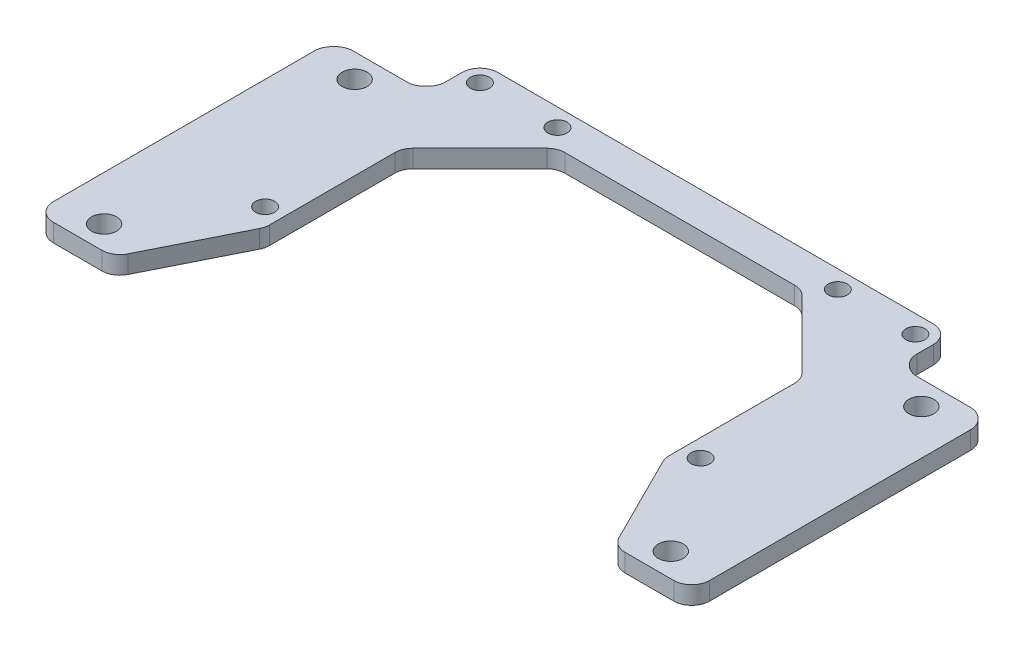
from build123d import *

# Parameters (mm, degrees)
SKETCH_1_R      = 2.1
SKETCH_1_R_2    = 1.6
EXTRUDE_1_DEPTH = 3
CHAMFER_1_SIZE  = 13
CHAMFER_2_SIZE  = 2
FILLET_1_R      = 3


with BuildPart() as part:
    # 草图1 → 凸台-拉伸1 (new body)
    with BuildSketch(Plane(origin=(0, 0, 0), x_dir=(1, 0, 0), z_dir=(0, 1, 0))):
        Polygon((-55, -25), (-55, 25), (-39.5, 25), (-39.5, 34), (39.5, 34), (39.5, 25), (55, 25), (55, -25), (42, -25), (33.5, -8), (33.5, 28), (0, 28), (-33.5, 28), (-33.5, -8), (-42, -25), align=None)
        with Locations(Location((-47.5, 21, 0), (0, 0, 270))):
            Circle(SKETCH_1_R, mode=Mode.SUBTRACT)
        with Locations(Location((-47.5, -21, 0), (0, 0, 270))):
            Circle(SKETCH_1_R, mode=Mode.SUBTRACT)
        with Locations(Location((47.5, -21, 0), (0, 0, 270))):
            Circle(SKETCH_1_R, mode=Mode.SUBTRACT)
        with Locations(Location((47.5, 21, 0), (0, 0, 270))):
            Circle(SKETCH_1_R, mode=Mode.SUBTRACT)
        with Locations(Location((-36.5, 31, 0), (0, 0, 270))):
            Circle(SKETCH_1_R_2, mode=Mode.SUBTRACT)
        with Locations(Location((-36.5, -5, 0), (0, 0, 270))):
            Circle(SKETCH_1_R_2, mode=Mode.SUBTRACT)
        with Locations(Location((36.5, -5, 0), (0, 0, 270))):
            Circle(SKETCH_1_R_2, mode=Mode.SUBTRACT)
        with Locations(Location((36.5, 31, 0), (0, 0, 270))):
            Circle(SKETCH_1_R_2, mode=Mode.SUBTRACT)
        with Locations(Location((-23.5, 31, 0), (0, 0, 270))):
            Circle(SKETCH_1_R_2, mode=Mode.SUBTRACT)
        with Locations(Location((23.5, 31, 0), (0, 0, 270))):
            Circle(SKETCH_1_R_2, mode=Mode.SUBTRACT)
    extrude(amount=EXTRUDE_1_DEPTH)

    # 倒角1
    chamfer_1_edges = [part.edges().sort_by_distance(p)[0] for p in [
        (33.5, 1.5, -28),
        (-33.5, 1.5, -28),
    ]]
    chamfer(chamfer_1_edges, length=CHAMFER_1_SIZE)

    # 倒角2
    chamfer_2_edges = [part.edges().sort_by_distance(p)[0] for p in [
        (55, 1.5, -25),
        (-55, 1.5, -25),
        (-39.5, 1.5, -25),
        (39.5, 1.5, -25),
    ]]
    chamfer(chamfer_2_edges, length=CHAMFER_2_SIZE)

    # 圆角1
    fillet_1_edges = [part.edges().sort_by_distance(p)[0] for p in [
        (41.5, 1.5, -25),
        (53, 1.5, -25),
        (55, 1.5, -23),
        (39.5, 1.5, -27),
        (-55, 1.5, -23),
        (-41.5, 1.5, -25),
        (-53, 1.5, -25),
        (-39.5, 1.5, -27),
        (55, 1.5, 25),
        (42, 1.5, 25),
        (33.5, 1.5, 8),
        (-33.5, 1.5, 8),
        (-42, 1.5, 25),
        (-55, 1.5, 25),
        (-39.5, 1.5, -34),
        (39.5, 1.5, -34),
        (33.5, 1.5, -15),
        (-20.5, 1.5, -28),
        (20.5, 1.5, -28),
        (-33.5, 1.5, -15),
    ]]
    fillet(fillet_1_edges, radius=FILLET_1_R)


solid = part.part
